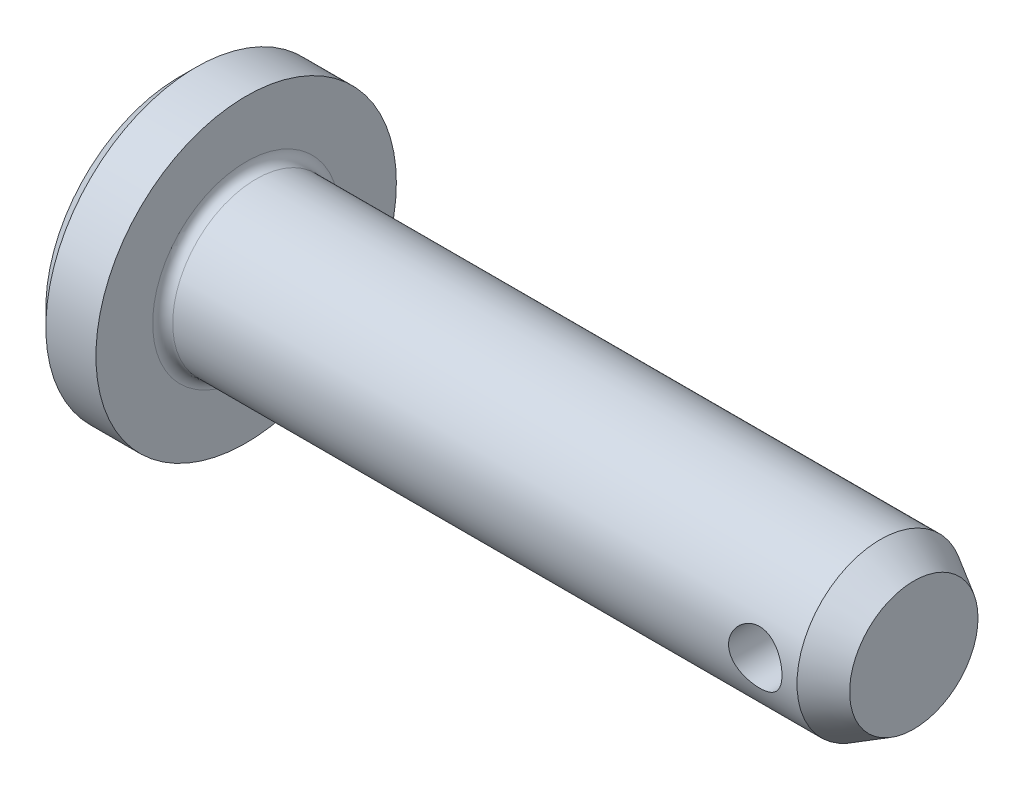
from build123d import *

# Parameters (mm, degrees)
CUT_EXTRUDE1_DEPTH      = 46.803929962
CUT_EXTRUDE1_DEPTH_BACK = 46.803929962
SKETCH2_R               = 1.6
FILLET1_R               = 0.6
CHAMFER1_SIZE           = 2
CHAMFER1_SIZE2          = 1.154700538


with BuildPart() as part:
    # Sketch1 → Base-Revolve (revolve)
    with BuildSketch(Plane.XY, mode=Mode.PRIVATE) as base_revolve_sk:
        Polygon((0, 0), (44, 0), (44, 5), (4, 5), (4, 9), (1, 9), (0, 8), align=None)
    revolve(base_revolve_sk.sketch.rotate(Axis((0, 0, 0), (-1, 0, 0)), 90), axis=Axis((0, 0, 0), (-1, 0, 0)))

    # Sketch2 → Cut-Extrude1 (cut, two sides: drawn at the far end of the back side and taken through both)
    with BuildSketch(Plane.XY.offset(-CUT_EXTRUDE1_DEPTH_BACK)):
        with Locations((39.5, 0)):
            Circle(SKETCH2_R)
    extrude(amount=CUT_EXTRUDE1_DEPTH + CUT_EXTRUDE1_DEPTH_BACK, mode=Mode.SUBTRACT)

    # Fillet1
    fillet1_edges = [part.edges().sort_by_distance(p)[0] for p in [
        (4, 0, 5),
    ]]
    fillet(fillet1_edges, radius=FILLET1_R)

    # Chamfer1
    chamfer1_edges = [part.edges().sort_by_distance(p)[0] for p in [
        (44, 0, 5),
    ]]
    chamfer1_side = [part.faces().sort_by_distance(p)[0] for p in [
        (24.3, 0, 5),
    ]]
    chamfer(chamfer1_edges, length=CHAMFER1_SIZE, length2=CHAMFER1_SIZE2, reference=chamfer1_side[0])


solid = part.part
